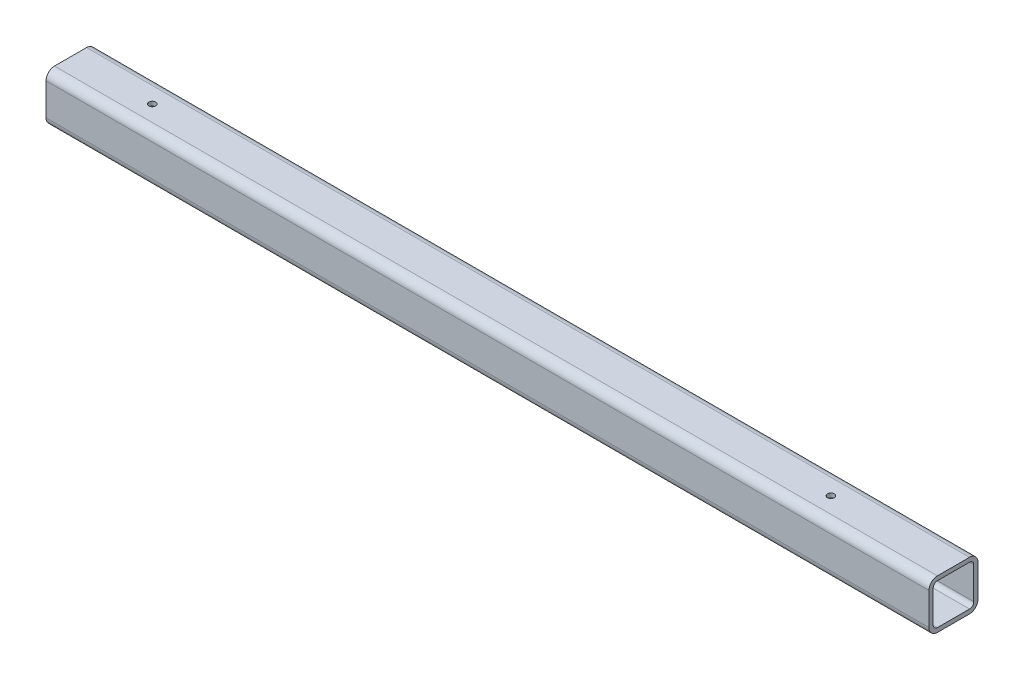
from build123d import *

# Parameters (mm, degrees)
MEMBER_1_DEPTH     = 540
HOLE_WIZARD_M5_1_D = 4.2
HOLE_WIZARD_2_D    = 4.2


with BuildPart() as part:
    # Sketch1 → Member 1 (new body)
    with BuildSketch(Plane(origin=(0, 0, 0), x_dir=(0, 0, -1), z_dir=(1, 0, 0))):
        with BuildLine():
            Line((-9.8, -15), (9.8, -15))
            ThreePointArc((9.8, -15), (13.476955262, -13.476955262), (15, -9.8))
            Line((15, -9.8), (15, 9.8))
            ThreePointArc((15, 9.8), (13.476955262, 13.476955262), (9.8, 15))
            Line((9.8, 15), (-9.8, 15))
            ThreePointArc((-9.8, 15), (-13.476955262, 13.476955262), (-15, 9.8))
            Line((-15, 9.8), (-15, -9.8))
            ThreePointArc((-15, -9.8), (-13.476955262, -13.476955262), (-9.8, -15))
        make_face()
        with BuildLine():
            Line((-9.8, -12.4), (9.8, -12.4))
            ThreePointArc((9.8, -12.4), (11.638477631, -11.638477631), (12.4, -9.8))
            Line((12.4, -9.8), (12.4, 9.8))
            ThreePointArc((12.4, 9.8), (11.638477631, 11.638477631), (9.8, 12.4))
            Line((9.8, 12.4), (-9.8, 12.4))
            ThreePointArc((-9.8, 12.4), (-11.638477631, 11.638477631), (-12.4, 9.8))
            Line((-12.4, 9.8), (-12.4, -9.8))
            ThreePointArc((-12.4, -9.8), (-11.638477631, -11.638477631), (-9.8, -12.4))
        make_face(mode=Mode.SUBTRACT)
    extrude(amount=MEMBER_1_DEPTH)

    # M5 螺纹孔1 (through all)
    with Locations(Plane(origin=(0, -15, 0), x_dir=(-1, 0, 0), z_dir=(0, -1, 0))):
        with Locations((-465, 0)):
            Hole(HOLE_WIZARD_M5_1_D / 2)

    # Hole Wizard 2 (through all)
    with Locations(Plane(origin=(0, -15, 0), x_dir=(-1, 0, 0), z_dir=(0, -1, 0))):
        with Locations((-50, 0)):
            Hole(HOLE_WIZARD_2_D / 2)


solid = part.part
